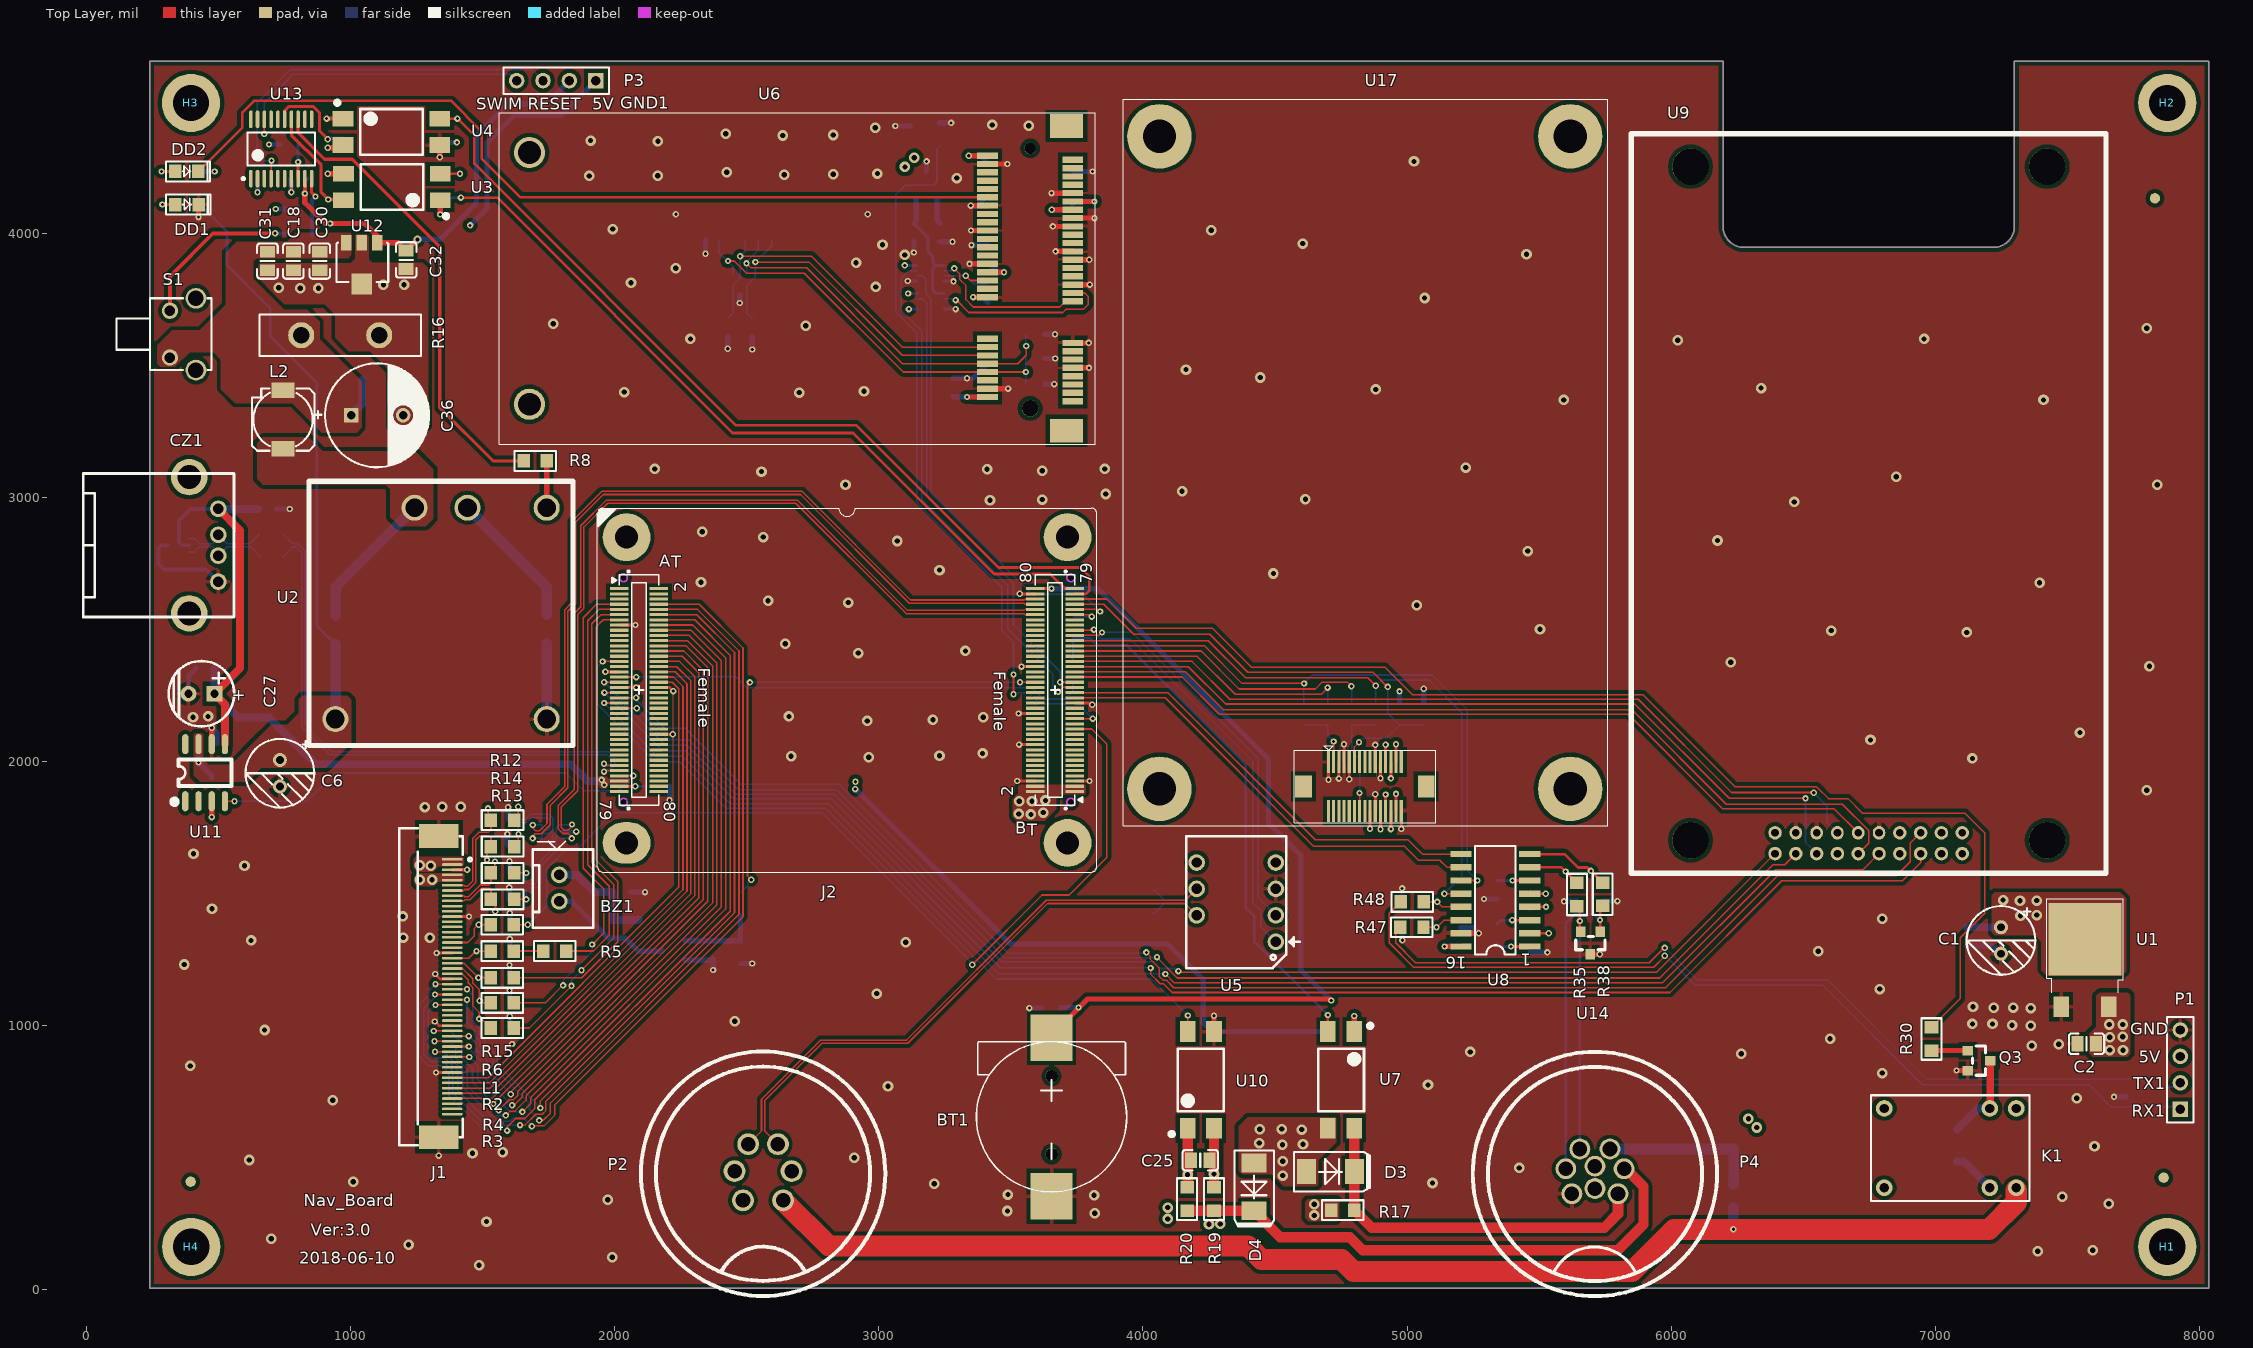
[diagram p0: Top Layer view]
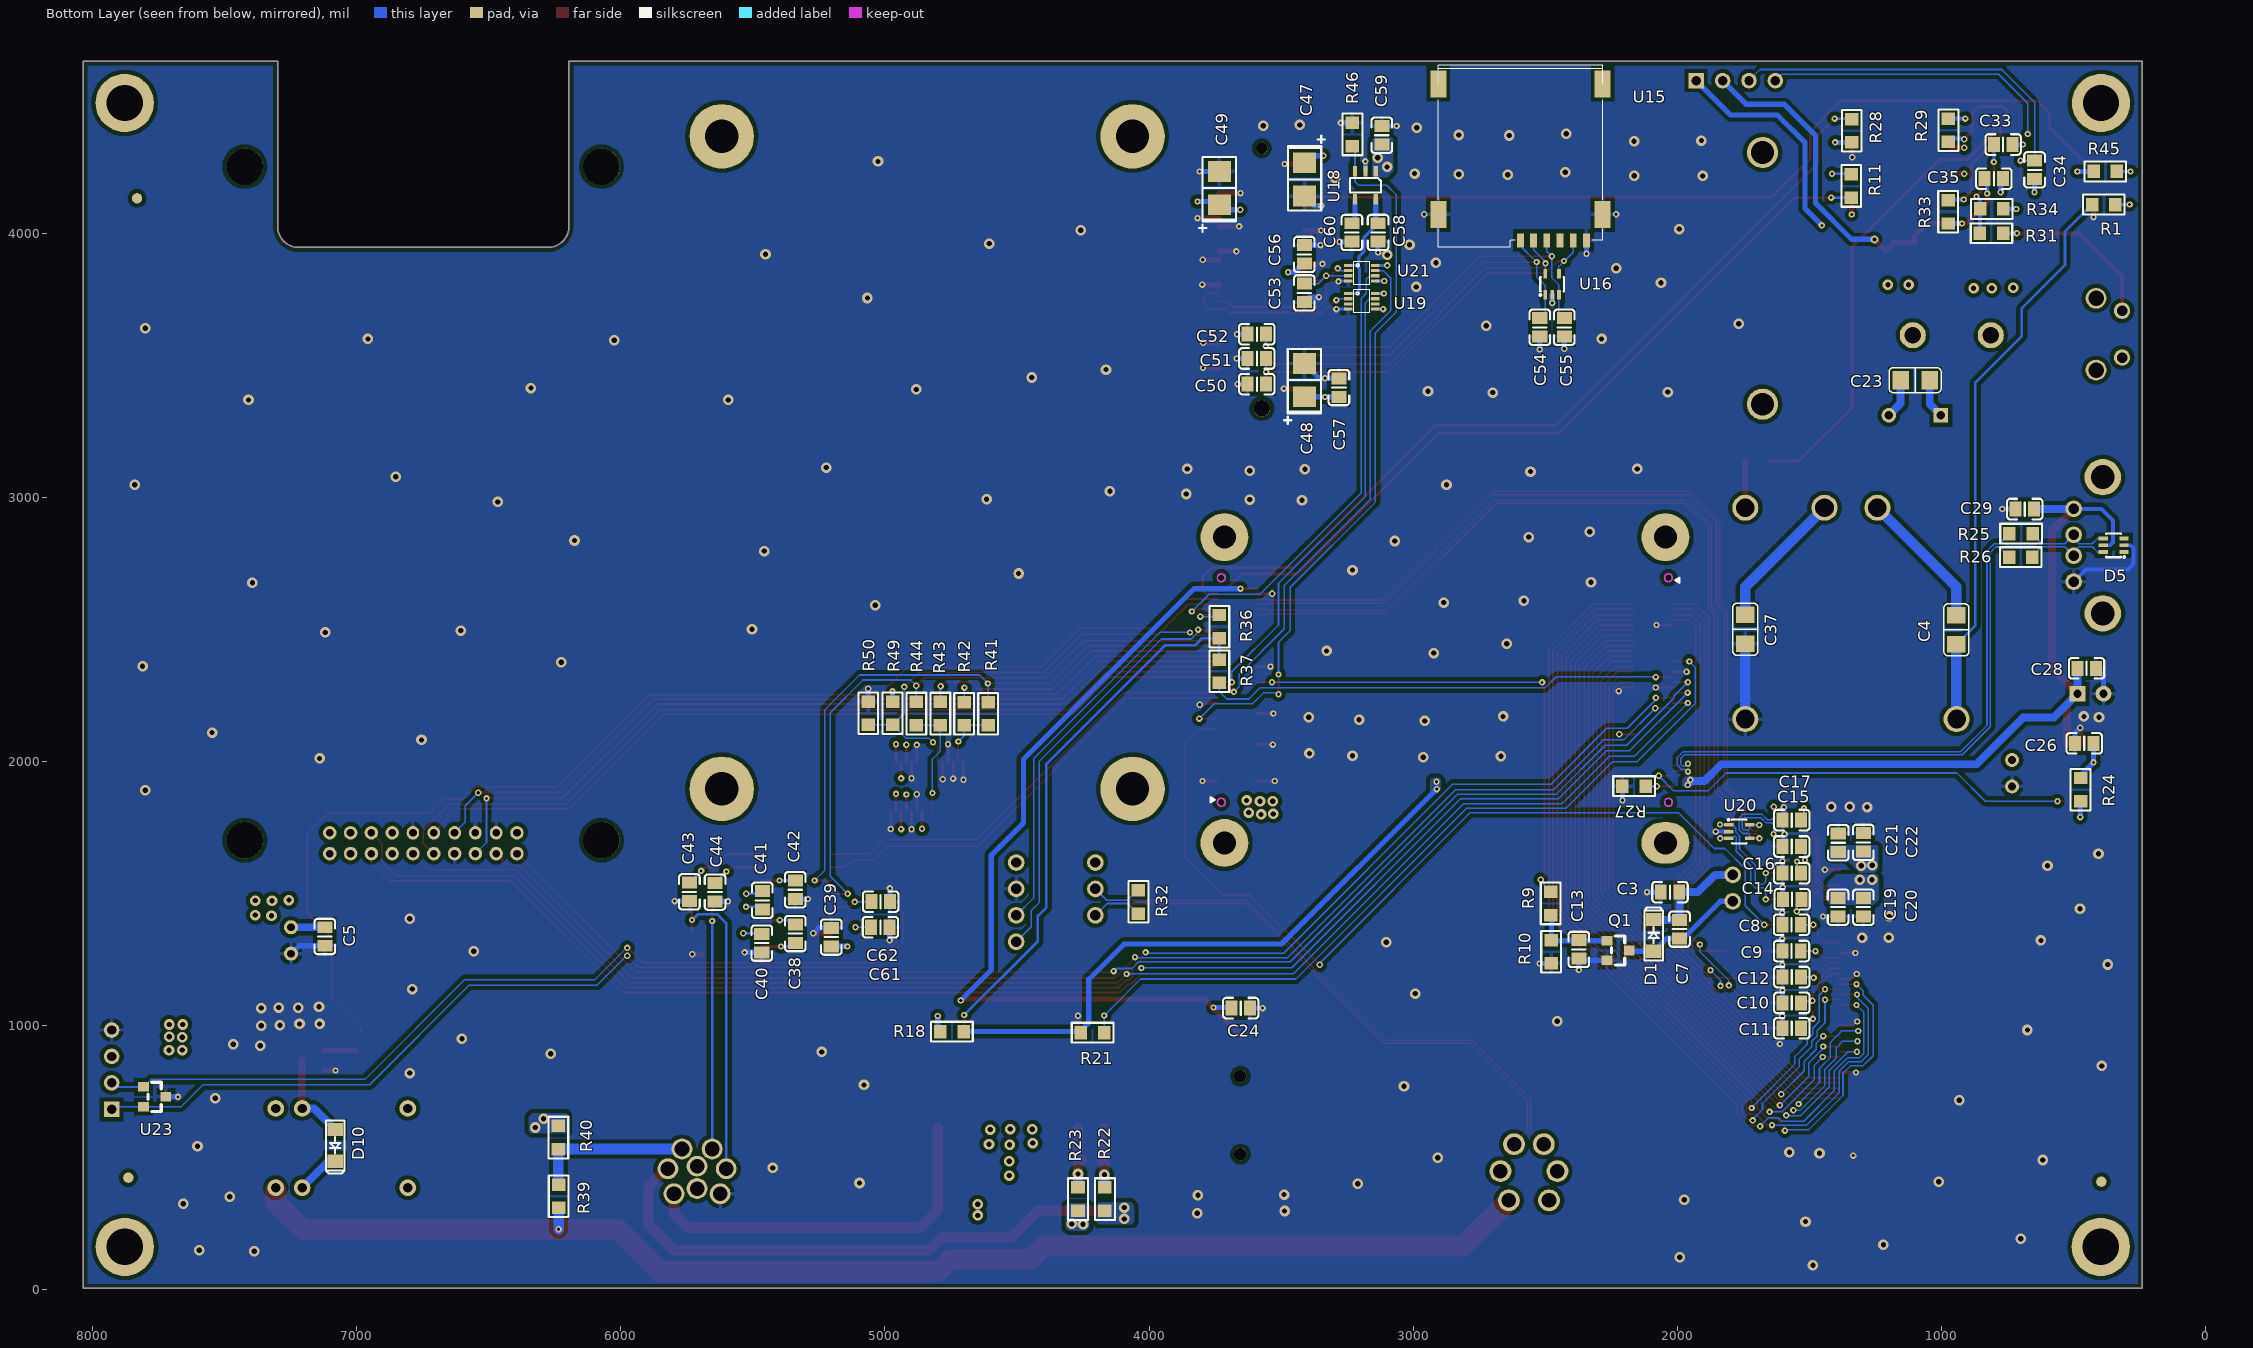
[diagram p1: Bottom Layer view, seen from below]
# Altium PCB MISC82794.PcbDoc (part 1 of 5)
Units mil, origin at the board's own origin, x right, y up, seen from the top; angles counter-clockwise.
Board outline 7795.28 x 4645.67 mil, 4 copper layers (Top Layer, GND, POWER, Bottom Layer); 157 components, 133 nets, 768 pads, 456 vias.

## Layer stack, top to bottom (the 12.6 mil dielectric is the usual default, probably not edited)
Top Layer: signal copper 1.4
Dielectric: core 12.6, FR-4, Dk 4.8
GND: plane copper 1.4, net GND
Dielectric: prepreg 12.6, FR-4, Dk 4.8
POWER: plane copper 1.4, net (Multiple Nets)
Dielectric: core 12.6, FR-4, Dk 4.8
Bottom Layer: signal copper 1.4

## Board outline
239.55,5.82 239.55,4651.49 6196.25,4651.49 6196.25,4025.5 ccw(c6274.99,4025.5) 6274.99,3946.76 7219.87,3946.76 ccw(c7219.87,4025.5) 7298.61,4025.5 7298.61,4651.49 8034.83,4651.49 8034.83,5.82

## Design rules (kind name [scope] priority, off if disabled: settings)
Clearance Clearance_1 [InPolygon] p1: gap=6
Clearance [All] p2: gap=6
ComponentClearance [All] p1 off: gap=10 collisioncheckmode=3 verticalgap=10 showdistances=FALSE
DiffPairsRouting [All] p1: maxlimit=6 minlimit=6 mostfreqgap=6 maxuncoupledlength=500
Height [All] p1: minheight=0 maxheight=70503.27 prefheight=500
HoleSize [All] p1: absolutevalues=TRUE maxlimit=10000 minlimit=1 maxpercent=80.000 minpercent=20.000
HoleToHoleClearance [All] p1: gap=0 allowstackedmicrovias=TRUE
MinimumSolderMaskSliver [All] p1 off: minsoldermaskwidth=10
PlaneClearance [All] p1: clearance=20
PlaneConnect [All] p1: planeconnectstyle=Direct reliefexpansion=20 reliefentries=4 reliefconductorwidth=10 reliefairgap=10
PolygonConnect PolygonConnect_2 [All vs isvia] p1: connectstyle=Direct reliefconductorwidth=10 reliefentries=4 polygonreliefangle="90 Angle"
PolygonConnect PolygonConnect_1 [InNet(GND)] p2: connectstyle=Relief reliefconductorwidth=15 reliefentries=4 polygonreliefangle="90 Angle"
PolygonConnect [All] p3: connectstyle=Direct reliefconductorwidth=10 reliefentries=4 polygonreliefangle="90 Angle"
RoutingVias [All] p1: holewidth=12 width=24 viastyle="Through Hole" minholewidth=12 minwidth=24 maxholewidth=12 maxwidth=24
SilkToSilkClearance [All] p1 off: silktosilkclearance=10
SilkscreenOverComponentPads [IsPad] p1 off: minsilkscreentomaskgap=10
SolderMaskExpansion [All] p1: expansion=4
Width [All] p1: maxlimit=80 minlimit=6 preferedwidth=6 bottomlayer_maxwidth=40 minimp=50.000000 maximp=50.000000 favimp=50.000000
18 further rules are at their usual default settings.

## Classes and differential pairs
differential pair NewDifferentialPair5: +TS_YM -TS_YP
differential pair NewDifferentialPair4: +TS_XM -TS_XP
differential pair NewDifferentialPair3: +XM -XP
differential pair NewDifferentialPair2: +YM -YP
differential pair NewDifferentialPair1: +USB0_N -USB0_P
differential pair USB0_H: +USB0_H_P -USB0_H_N
differential pair NewDifferentialPair6: +CANH0 -CANL0

## Components (designator, comment, footprint, x,y, rotation, side; value= is the part's Value field where it differs from the comment)
BT1 "BATTERY" BATTERY-1220-1 3654,655 r0 top
BZ1 "BUZZER2" XH2.5-2P 1691,1671 r270 top
C1 "100μF/25V" RB6.3*7 7248,1323 r270 top
C2 "100nF" 0805C 7572,932 r180 top
C3 "100nF" 0805C 2028,1506 r0 bottom
C4 "1nF/2kV" C1206 944,2499 r270 bottom
C5 "100nF" 0805C 7120,1338 r270 bottom
C6 "100μF/25V" RB6.3*7 733,1956 r270 top
C7 "100nF" 0805C 1992,1366 r90 bottom
C8 "15PF,±5%" 0805C 1568,1382.6 r0 bottom
C9 "15PF,±5%" 0805C 1568,1283 r0 bottom
C10 "15PF,±5%" 0805C 1567,1086.6 r0 bottom
C11 "15PF,±5%" 0805C 1567,990.6 r0 bottom
C12 "15PF,±5%" 0805C 1567,1184.6 r0 bottom
C13 "100nF" 0805C 2373,1289 r90 bottom
C14 "1nF,CAP" 0805C 1566,1478.6 r0 bottom
C15 "1nF,CAP" 0805C 1567,1678.6 r0 bottom
C16 "1nF,CAP" 0805C 1567,1577.6 r0 bottom
C17 "1nF,CAP" 0805C 1567,1778.6 r0 bottom
C18 "100nF" 0805C 784,3895 r270 top
C19 "100nF" 0805C 1392,1449 r90 bottom
C20 "10μF 10V" 0805C 1296,1449 r90 bottom
C21 "10μF 10V" 0805C 1391,1693 r90 bottom
C22 "100nF" 0805C 1296,1694 r270 bottom
C23 "4.7uF/25V" C1206 1100,3444 r180 bottom
C24 "100nF" 0805C 3653,1067 r180 bottom
C25 "1μF,±10%" 0805C 4217,491 r0 top
C26 "100nF" 0805C 460,2069 r180 bottom
C27 "100μF,25V" CAPPRD250W45D630H800P 436,2257 r180 top
C28 "10μF 10V" 0805C 451,2353 r180 bottom
C29 "100nF" 0805C 685,2956 r0 bottom
C30 "100nF" 0805C 884,3895 r270 top
C31 "100nF" 0805C 686,3895 r270 top
C32 "100nF" 0805C 1211,3899 r270 top
C33 "1uF" 0805C 767,4336 r0 bottom
C34 "100nF" 0805C 648,4240 r90 bottom
C35 "100nF" 0805C 801.98,4206.79 r180 bottom
C36 "330μF/35V" CAPPR5.0-10X16-0.8 1101,3311 r0 top
C37 "1nF/2kV" C1206 1743,2501 r270 bottom
C38 "100nF" 0805C 5339,1349 r270 bottom
C39 "100nF" 0805C 5203,1336 r90 bottom
C40 "100nF" 0805C 5466,1313 r270 bottom
C41 "100nF" 0805C 5464,1475 r270 bottom
C42 "100nF" 0805C 5339,1515 r270 bottom
C43 "15pF" 0805C 5740,1507 r270 bottom
C44 "15pF" 0805C 5643,1506 r270 bottom
C47 "150μF/6.3V" CT3528-B 3411,4204 r270 bottom
C48 "150μF/6.3V" CT3528-B 3412,3444 r90 bottom
C49 "150μF/6.3V" CT3528-B 3734,4171 r90 bottom
C50 "1μF" 0805C 3592,3429 r0 bottom
C51 "33pF" 0805C 3592,3526 r0 bottom
C52 "33pF" 0805C 3592,3618 r0 bottom
C53 "33pF" 0805C 3412,3774 r270 bottom
C54 "33pF" 0805C 2521,3644 r90 bottom
C55 "33pF" 0805C 2428,3644 r90 bottom
C56 "100nF" 0805C 3412,3920 r90 bottom
C57 "10pF" 0805C 3281,3416 r90 bottom
C58 "1μF,±10%" 0805C 3133,4003 r90 bottom
C59 "1μF,±10%" 0805C 3119,4371 r270 bottom
C60 "22nF,±10%" 0805C 3232,4003 r90 bottom
C61 "15pF" 0805C 5017,1373 r0 bottom
C62 "15pF" 0805C 5016,1470 r0 bottom
CZ1 "USB" USB-1400 445,2819 r180 top
D1 "1N4148" SMD-D4148 2090,1342 r90 bottom
D3 "P6SMB15A" DO-214 4710,448 r0 top
D4 "P6SMB15A" DO-214 4421,390 r270 top
D5 "NUP4202W1" SOT-363 349,2819 r0 bottom
D10 "1N4148" SMD-D4148 7081,547 r270 bottom
DD1 "RED 0603" LED0805 381.14,4108.86 r0 top
DD2 "RED 0603" LED0805 380,4234 r0 top
H1 "Hole" HOLE-3.2#1 7877,163 r0 top
H2 "Hole" HOLE-3.2#2 7840,4365 r0 top
H3 "Hole" HOLE-3.2#3 609,4505 r0 top
H4 "Hole" HOLE-3.2#1 397,163 r0 top
J1 "FPC-50" FFC0.5-50P-A 1360,1148 r270 top locked
J2 "HEADER 40X2" AM3352B 2880,2271 r0 top locked
K1 "HK4100F-DC5V-SHG 0.2W" HK4100F 7306,687 r180 top
L1 "1nH" 0805R 1575,1282.6 r180 top
L2 "4.7uH" SLF6045 627,3413 r270 top
P1 "2.54 single-row header-4pin" HDR1X4 7927,684 r90 top
P2 "6-core" BBD-06PMFP-LC7001 2562,440 r180 top locked
P3 "2.54 single-row header-4pin" HDR1X4 1929,4578 r180 top
P4 "8-core" BDU-08PMFP-LC7001 5711,439 r180 top locked
Q1 "SS8050LT(1.5A)" SOT-23 2224,1285 r180 bottom
Q3 "SS8050LT(1.5A)" SOT-23 7165,868 r0 top
R1 "2KΩ 1%" 0805R 386.14,4108.86 r0 bottom
R2 "22Ω,±5%" 0805R 1575,1181.6 r180 top
R3 "22Ω,±5%" 0805R 1575,991.6 r180 top
R4 "22Ω,±5%" 0805R 1575,1086.6 r180 top
R5 "22Ω,±5%" 0805R 1773,1283 r180 top
R6 "22Ω,±5%" 0805R 1575,1382.6 r180 top
R8 "0Ω,±5%" 0805R 1700,3138 r180 top
R9 "4.7K  1%" 0805R 2480,1463 r270 bottom
R10 "4.7K  1%" 0805R 2478,1280 r90 bottom
R11 "1kΩ,±1%" 0805R 1342,4179 r90 bottom
R12 "0Ω,±5%" 0805R 1576,1778.6 r180 top
R13 "0Ω,±5%" 0805R 1576,1578.6 r180 top
R14 "0Ω,±5%" 0805R 1576,1678.6 r180 top
R15 "0Ω,±5%" 0805R 1576,1478.6 r180 top
R16 "14D560K" 14D560K 1109,3614 r90 top
R17 "10kΩ,±1%" 0805R 4756,302 r180 top
R18 "2KΩ 1%" 0805R 4746,978 r0 bottom
R19 "2KΩ 1%" 0805R 4269,344 r90 top
R20 "2KΩ 1%" 0805R 4167,344 r90 top
R21 "10kΩ,±1%" 0805R 4214,974 r180 bottom
R22 "10KΩ,±1%" 0805R 4167,344 r270 bottom
R23 "10KΩ,±1%" 0805R 4269,344 r270 bottom
R24 "10KΩ,±1%" 0805R 474,1894 r90 bottom
R25 "22Ω,±5%" 0805R 699,2863 r180 bottom
R26 "22Ω,±5%" 0805R 700,2774 r180 bottom
R27 "1KΩ,±1%" 0805R 2164,1907 r180 bottom
R28 "10KΩ,±1%" 0805R 1340,4388 r90 bottom
R29 "2KΩ 1%" 0805R 974,4390 r270 bottom
R30 "1kΩ,±1%" 0805R 6985,950 r270 top
R31 "10KΩ,±1%" 0805R 811,4000 r0 bottom
R32 "120Ω 1%" 0805R 4040,1469 r90 bottom
R33 "10KΩ,±1%" 0805R 975,4081 r90 bottom
R34 "4.7K  1%" 0805R 810,4092 r0 bottom
R35 "4.7Ω,±1%" 0805R 5643,1497 r90 top
R36 "0Ω,±5%" 0805R 3734,2511 r90 bottom
R37 "0Ω,±5%" 0805R 3734,2342 r270 bottom
R38 "4.7Ω,±1%" 0805R 5740,1498 r90 top
R39 "0Ω,±1%" 0805R 6235,355 r270 bottom
R40 "0Ω,±1%" 0805R 6236,577 r90 bottom
R41 "0Ω,±5%" 0805R 4609,2181 r270 bottom
R42 "0Ω,±5%" 0805R 4700,2181 r270 bottom
R43 "0Ω,±5%" 0805R 4790,2182 r270 bottom
R44 "0Ω,±5%" 0805R 4881,2182 r270 bottom
R45 "470Ω,±1%" 0805R 380,4234 r180 bottom
R46 "100K" 0805R 3230,4374 r90 bottom
R47 "4.7Ω,±1%" 0805R 5018,1373 r0 top
R48 "4.7Ω,±1%" 0805R 5019,1469 r0 top
R49 "10KΩ,±1%" 0805R 4971,2183 r90 bottom
R50 "10KΩ,±1%" 0805R 5063,2183 r90 bottom
S1 "SW-PB4P" SWICH4.5 366,3618 r90 top
U1 "LD1086DT33TR" DPAK 7566,1200 r0 top
U2 "E2405UHBDD-10W" E2403UHBDD 1343,2561 r270 top
U3 "PC817" SMD-4 1157,4175 r180 top
U4 "PC817" SMD-4 1155,4384 r0 top
U5 "CTM1051AM" CTM1051AM 4353,1468 r90 top
U6 "ME909s-821" PCIE_0 3573,3337 r90 top locked
U7 "PC817" SMD-4 4750,795 r270 top
U8 "SP3232EEN" SOP16-6.6 5334,1475 r180 top
U9 "2.0mm dual-row socket-20pin" 20PIN-OEM_STARA 6748,2952 r180 top locked
U10 "PC817" SMD-4 4219,795 r90 top
U11 "SP2526A" SOIC127P600X175-8N 450,1958 r90 top
U12 "78L05M" SOT-89 1043,3886 r180 top
U13 "STM8S103F3" TSOP65P640X120-20N 738,4319 r90 top
U14 "PESD15VL2BT" SOT-23 5694,1313 r270 top
U15 "USIM" SIM 2594,4269 r0 bottom
U16 "PESD3V3L4UG" SOT-353 2474,3807 r90 bottom
U17 "HX-DU1006D" HX-DU1006D 4840,1906 r180 top locked
U18 "RT9193-18GB" SOT23-5 3181,4182 r0 bottom
U19 "SN74LVC2T45" VSSOP-8 3195.26,3742.47 r180 bottom
U20 "PESD3V3L4UG" SOT-353 1766,1735 r180 bottom
U21 "SN74LVC2T45" VSSOP-8 3195,3849 r180 bottom
U23 "PESD15VL2BT" SOT-23 7764,731 r180 bottom

## Footprints (in the part's own frame and the unit in brackets; to place one, negate y for a bottom-side part, rotate by r counter-clockwise, add the part's x,y. Pads: shape width x height; smd on the part's side, far side on the other; paste and mask are expansions set on the pad)
14D560K [mm]
  round 2.5 hole 1.6: 1(0,0) 2(0,7.5)
  silkscreen extent -2,-4 2,11.5
20PIN-OEM_STARA [mm]
  round 1.3 hole 0.737: 1(-8.975,33.025) 2(-8.975,31.025) 3(-6.975,33.025) 4(-6.975,31.025) 5(-4.975,33.025) 6(-4.975,31.025) 7(-2.975,33.025) 8(-2.975,31.025) 9(-0.975,33.025) 11(1.025,33.025) 13(3.025,33.025) 15(5.025,33.025) 17(7.025,33.025) 19(9.025,33.025) 20(9.025,31.025)
  oval 1.2x1.3 hole 0.737: 10(-0.975,31.025) 12(1.025,31.025) 14(3.025,31.025) 16(5.025,31.025) 18(7.025,31.025)
  round 3.5 hole 3.5: 21(17.145,-33.025) 22(17.145,31.745) 23(-17.145,-33.025) 24(-17.145,31.745)
  silkscreen extent -22.8,-36.18 22.86,34.92
0805C [mm]
  rect 1.15x1.45 smd: 1(-0.889,0) 2(0.889,0)
  silkscreen extent -1.7,-0.99 1.7,0.99, body extent -1,-0.63 1,0.63, height 0.78
0805R [mm]
  rect 1.2x1.3 smd: 1(-1.118,0) 2(1.118,0)
  silkscreen extent -2,-0.95 2,0.95
AM3352B [mm]
  round 0.6 hole 0.6 unplated mask+0.254: 0(-21.5,-10.8) 0(-21.5,-10.8) 0(-21.5,10.8) 0(-21.5,10.8) 0(21.5,-10.8) 0(21.5,-10.8) 0(21.5,10.8) 0(21.5,10.8)
  round 4.6 hole 2.2: 1(-21.2,14.7) 3(21.2,14.7) 4(21.2,-14.7)
  oval 4.6x4 hole 2.2: 2(-21.2,-14.7)
  rect 1.8x0.3 smd: A1(-21.9,9.75) A2(-18.1,9.75) A3(-21.9,9.25) A4(-18.1,9.25) A5(-21.9,8.75) A6(-18.1,8.75) A7(-21.9,8.25) A8(-18.1,8.25) A9(-21.9,7.75) A10(-18.1,7.75) A11(-21.9,7.25) A12(-18.1,7.25) A13(-21.9,6.75) A14(-18.1,6.75) A15(-21.9,6.25) A16(-18.1,6.25) A17(-21.9,5.75) A18(-18.1,5.75) A19(-21.9,5.25) A20(-18.1,5.25) A21(-21.9,4.75) A22(-18.1,4.75) A23(-21.9,4.25) A24(-18.1,4.25) A25(-21.9,3.75) A26(-18.1,3.75) A27(-21.9,3.25) A28(-18.1,3.25) A29(-21.9,2.75) A30(-18.1,2.75) A31(-21.9,2.25) A32(-18.1,2.25) A33(-21.9,1.75) A34(-18.1,1.75) A35(-21.9,1.25) A36(-18.1,1.25) A37(-21.9,0.75) A38(-18.1,0.75) A39(-21.9,0.25) A40(-18.1,0.25) A41(-21.9,-0.25) A42(-18.1,-0.25) A43(-21.9,-0.75) A44(-18.1,-0.75) A45(-21.9,-1.25) A46(-18.1,-1.25) A47(-21.9,-1.75) A48(-18.1,-1.75) A49(-21.9,-2.25) A50(-18.1,-2.25) A51(-21.9,-2.75) A52(-18.1,-2.75) A53(-21.9,-3.25) A54(-18.1,-3.25) A55(-21.9,-3.75) A56(-18.1,-3.75) A57(-21.9,-4.25) A58(-18.1,-4.25) A59(-21.9,-4.75) A60(-18.1,-4.75) A61(-21.9,-5.25) A62(-18.1,-5.25) A63(-21.9,-5.75) A64(-18.1,-5.75) A65(-21.9,-6.25) A66(-18.1,-6.25) A67(-21.9,-6.75) A68(-18.1,-6.75) A69(-21.9,-7.25) A70(-18.1,-7.25) A71(-21.9,-7.75) A72(-18.1,-7.75) A73(-21.9,-8.25) A74(-18.1,-8.25) A75(-21.9,-8.75) A76(-18.1,-8.75) A77(-21.9,-9.25) A78(-18.1,-9.25) A79(-21.9,-9.75) A80(-18.1,-9.75) B1(21.9,-9.75) B2(18.1,-9.75) B3(21.9,-9.25) B4(18.1,-9.25) B5(21.9,-8.75) B6(18.1,-8.75) B7(21.9,-8.25) B8(18.1,-8.25) B9(21.9,-7.75) B10(18.1,-7.75) B11(21.9,-7.25) B12(18.1,-7.25) B13(21.9,-6.75) B14(18.1,-6.75) B15(21.9,-6.25) B16(18.1,-6.25) B17(21.9,-5.75) B18(18.1,-5.75) B19(21.9,-5.25) B20(18.1,-5.25) B21(21.9,-4.75) B22(18.1,-4.75) B23(21.9,-4.25) B24(18.1,-4.25) B25(21.9,-3.75) B26(18.1,-3.75) B27(21.9,-3.25) B28(18.1,-3.25) B29(21.9,-2.75) B30(18.1,-2.75) B31(21.9,-2.25) B32(18.1,-2.25) B33(21.9,-1.75) B34(18.1,-1.75) B35(21.9,-1.25) B36(18.1,-1.25) B37(21.9,-0.75) B38(18.1,-0.75) B39(21.9,-0.25) B40(18.1,-0.25) B41(21.9,0.25) B42(18.1,0.25) B43(21.9,0.75) B44(18.1,0.75) B45(21.9,1.25) B46(18.1,1.25) B47(21.9,1.75) B48(18.1,1.75) B49(21.9,2.25) B50(18.1,2.25) B51(21.9,2.75) B52(18.1,2.75) B53(21.9,3.25) B54(18.1,3.25) B55(21.9,3.75) B56(18.1,3.75) B57(21.9,4.25) B58(18.1,4.25) B59(21.9,4.75) B60(18.1,4.75) B61(21.9,5.25) B62(18.1,5.25) B63(21.9,5.75) B64(18.1,5.75) B65(21.9,6.25) B66(18.1,6.25) B67(21.9,6.75) B68(18.1,6.75) B69(21.9,7.25) B70(18.1,7.25) B71(21.9,7.75) B72(18.1,7.75) B73(21.9,8.25) B74(18.1,8.25) B75(21.9,8.75) B76(18.1,8.75) B77(21.9,9.25) B78(18.1,9.25) B79(21.9,9.75) B80(18.1,9.75)
  Keep-Out Layer circle w0.127: c21.5,10.8 r0.38
  Keep-Out Layer circle w0.127: c21.5,-10.8 r0.38
  Keep-Out Layer circle w0.127: c-21.5,-10.8 r0.38
  Keep-Out Layer circle w0.127: c-21.5,-10.8 r0.38
  Keep-Out Layer circle w0.127: c21.5,-10.8 r0.38
  Keep-Out Layer circle w0.127: c-21.5,10.8 r0.38
  Keep-Out Layer circle w0.127: c-21.5,10.8 r0.38
  silkscreen extent -24,-17.5 24,17.5